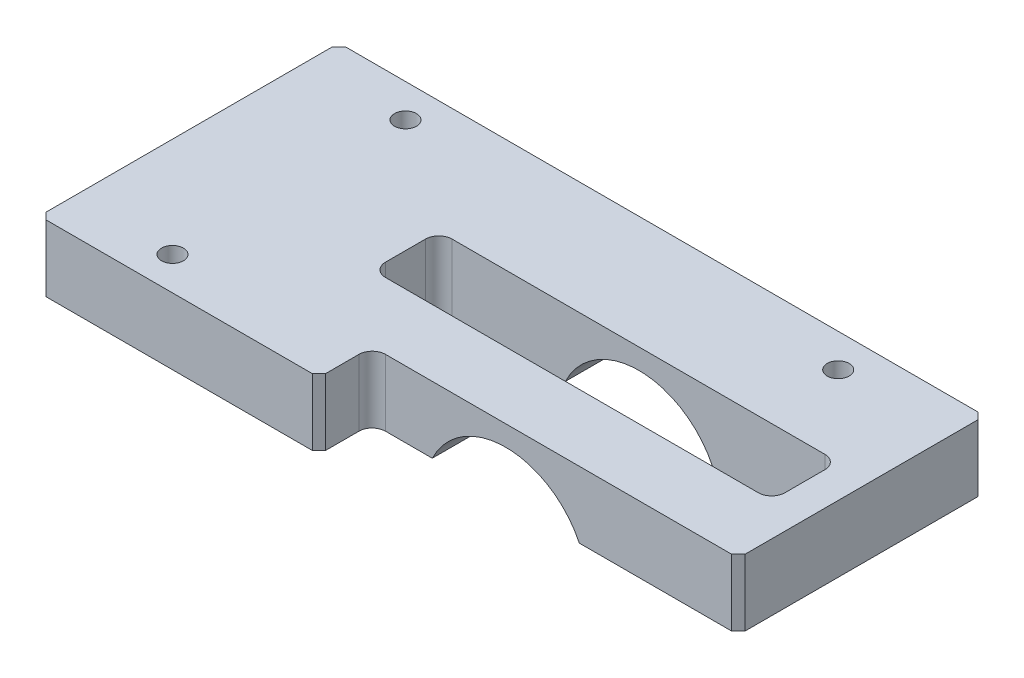
from build123d import *

# Parameters (mm, degrees)
SKETCH1_W             = 290
SKETCH1_H             = 45
BOSS_EXTRUDE1_DEPTH   = 10
SKETCH3_W             = 60
SKETCH3_H             = 10
CUT_EXTRUDE2_DEPTH    = 10
SKETCH4_W             = 45
SKETCH4_H             = 10
BOSS_EXTRUDE2_DEPTH   = 22
SKETCH6_R             = 5
CUT_EXTRUDE4_DEPTH    = 30
SKETCH7_W             = 80
SKETCH7_H             = 25
CUT_EXTRUDE5_DEPTH    = 27
SKETCH9_W             = 80
SKETCH9_H             = 45
CUT_EXTRUDE7_DEPTH    = 42
CUT_EXTRUDE8_DEPTH    = 20
SKETCH13_W            = 223.21076669
SKETCH13_H            = 10
CUT_EXTRUDE11_DEPTH   = 105
M5_TAPPED_HOLE1_D     = 4.2
M5_TAPPED_HOLE1_DEPTH = 12.4
M5_TAPPED_HOLE1_TIP   = 1.2618073
SKETCH19_W            = 55
SKETCH19_H            = 8
CUT_EXTRUDE13_DEPTH   = 169.805361289
SKETCH20_R            = 12.25
CUT_EXTRUDE14_DEPTH   = 174.245490562
M4_TAPPED_HOLE1_D     = 3.3
M4_TAPPED_HOLE1_DEPTH = 10.1
M4_TAPPED_HOLE1_TIP   = 0.991420021
CHAMFER1_SIZE         = 1
FILLET1_R             = 2
FILLET2_R             = 2


with BuildPart() as part:
    # Sketch1 → Boss-Extrude1 (new body)
    with BuildSketch(Plane(origin=(0, 0, 0), x_dir=(1, 0, 0), z_dir=(0, 1, 0))):
        Rectangle(SKETCH1_W, SKETCH1_H)
    extrude(amount=BOSS_EXTRUDE1_DEPTH)

    # Sketch3 → Cut-Extrude2 (cut)
    with BuildSketch(Plane(origin=(0, 10, 0), x_dir=(1, 0, 0), z_dir=(0, 1, 0))):
        with Locations((-105, 0.5)):
            Rectangle(SKETCH3_W, SKETCH3_H)
    extrude(amount=-CUT_EXTRUDE2_DEPTH, mode=Mode.SUBTRACT)

    # Sketch4 → Boss-Extrude2 (add)
    with BuildSketch(Plane.ZY.offset(145)):
        with Locations((0, 5)):
            Rectangle(SKETCH4_W, SKETCH4_H)
    extrude(amount=BOSS_EXTRUDE2_DEPTH)

    # Sketch6 → Cut-Extrude4 (cut)
    with BuildSketch(Plane(origin=(0, 10, 0), x_dir=(1, 0, 0), z_dir=(0, 1, 0))):
        with Locations(Location((-10, 0.5, 0), (0, 0, 270))):
            Circle(SKETCH6_R)
        with Locations(Location((-50, 0.5, 0), (0, 0, 270))):
            Circle(SKETCH6_R)
    extrude(amount=-CUT_EXTRUDE4_DEPTH, mode=Mode.SUBTRACT)

    # Sketch7 → Cut-Extrude5 (cut)
    with BuildSketch(Plane.XZ):
        with Locations((-30, -0.5)):
            Rectangle(SKETCH7_W, SKETCH7_H)
    extrude(amount=-CUT_EXTRUDE5_DEPTH, mode=Mode.SUBTRACT)

    # Sketch9 → Cut-Extrude7 (cut)
    with BuildSketch(Plane(origin=(0, 10, 0), x_dir=(1, 0, 0), z_dir=(0, 1, 0))):
        with Locations((-30, 0)):
            Rectangle(SKETCH9_W, SKETCH9_H)
    extrude(amount=-CUT_EXTRUDE7_DEPTH, mode=Mode.SUBTRACT)


with BuildPart() as cut_extrude7_piece_1:
    # of the separate pieces the step leaves, piece 1, a body of its own (cut_extrude7_pieces)
    add(part.part.solids().sort_by_distance((145, 0, -22.5))[0])

    # Sketch10 → Cut-Extrude8 (cut)
    with BuildSketch(Plane.XY.offset(22.5)):
        Polygon((145, 0), (145, 5), (130, 0), align=None)
    extrude(amount=-CUT_EXTRUDE8_DEPTH, mode=Mode.SUBTRACT)

    # Sketch13 → Cut-Extrude11 (cut)
    with BuildSketch(Plane.XY.offset(22.5)):
        with Locations((41.605383345, 5)):
            Rectangle(SKETCH13_W, SKETCH13_H)
    extrude(amount=-CUT_EXTRUDE11_DEPTH, mode=Mode.SUBTRACT)


with BuildPart() as cut_extrude7_piece_2:
    # of the separate pieces the step leaves, piece 2, a body of its own (cut_extrude7_pieces)
    add(part.part.solids().sort_by_distance((-70, 10, -22.5))[0])

    # M5 Tapped Hole1
    with Locations(Plane(origin=(-159, 5, -22.5), x_dir=(-1, 0, 0), z_dir=(0, 0, -1))):
        with Locations((0, 0), (-78, 0)):
            Hole(M5_TAPPED_HOLE1_D / 2, depth=M5_TAPPED_HOLE1_DEPTH)
            with Locations((0, 0, -(M5_TAPPED_HOLE1_DEPTH + M5_TAPPED_HOLE1_TIP / 2))):  # 118° drill point
                Cone(0, M5_TAPPED_HOLE1_D / 2, M5_TAPPED_HOLE1_TIP, mode=Mode.SUBTRACT)

    # Sketch19 → Cut-Extrude13 (cut, through all)
    with BuildSketch(Plane(origin=(0, 10, 0), x_dir=(1, 0, 0), z_dir=(0, 1, 0))):
        with Locations((-97.5, -18.5)):
            Rectangle(SKETCH19_W, SKETCH19_H)
    extrude(amount=-CUT_EXTRUDE13_DEPTH, mode=Mode.SUBTRACT)

    # Sketch20 → Cut-Extrude14 (cut, through all)
    with BuildSketch(Plane.XY.offset(22.5)):
        with Locations((-104.93, -5.3)):
            Circle(SKETCH20_R)
    extrude(amount=-CUT_EXTRUDE14_DEPTH, mode=Mode.SUBTRACT)

    # M4 Tapped Hole1
    with Locations(Plane(origin=(-152, 10, -17.5), x_dir=(0, 0, 1), z_dir=(0, 1, 0))):
        with Locations((0, 0), (0, 65), (35, 0)):
            Hole(M4_TAPPED_HOLE1_D / 2, depth=M4_TAPPED_HOLE1_DEPTH)
            with Locations((0, 0, -(M4_TAPPED_HOLE1_DEPTH + M4_TAPPED_HOLE1_TIP / 2))):  # 118° drill point
                Cone(0, M4_TAPPED_HOLE1_D / 2, M4_TAPPED_HOLE1_TIP, mode=Mode.SUBTRACT)

    # Chamfer1
    chamfer1_edges = [cut_extrude7_piece_2.edges().sort_by_distance(p)[0] for p in [
        (-167, 5, -22.5),
        (-167, 5, 22.5),
        (-70, 5, 14.5),
        (-125, 5, 22.5),
        (-70, 5, -22.5),
    ]]
    chamfer(chamfer1_edges, length=CHAMFER1_SIZE)

    # Fillet1
    fillet1_edges = [cut_extrude7_piece_2.edges().sort_by_distance(p)[0] for p in [
        (-125, 5, 14.5),
    ]]
    fillet(fillet1_edges, radius=FILLET1_R)

    # Fillet2
    fillet2_edges = [cut_extrude7_piece_2.edges().sort_by_distance(p)[0] for p in [
        (-75, 5, 4.5),
        (-135, 5, 4.5),
        (-135, 5, -5.5),
        (-75, 5, -5.5),
    ]]
    fillet(fillet2_edges, radius=FILLET2_R)


solid = cut_extrude7_piece_2.part
